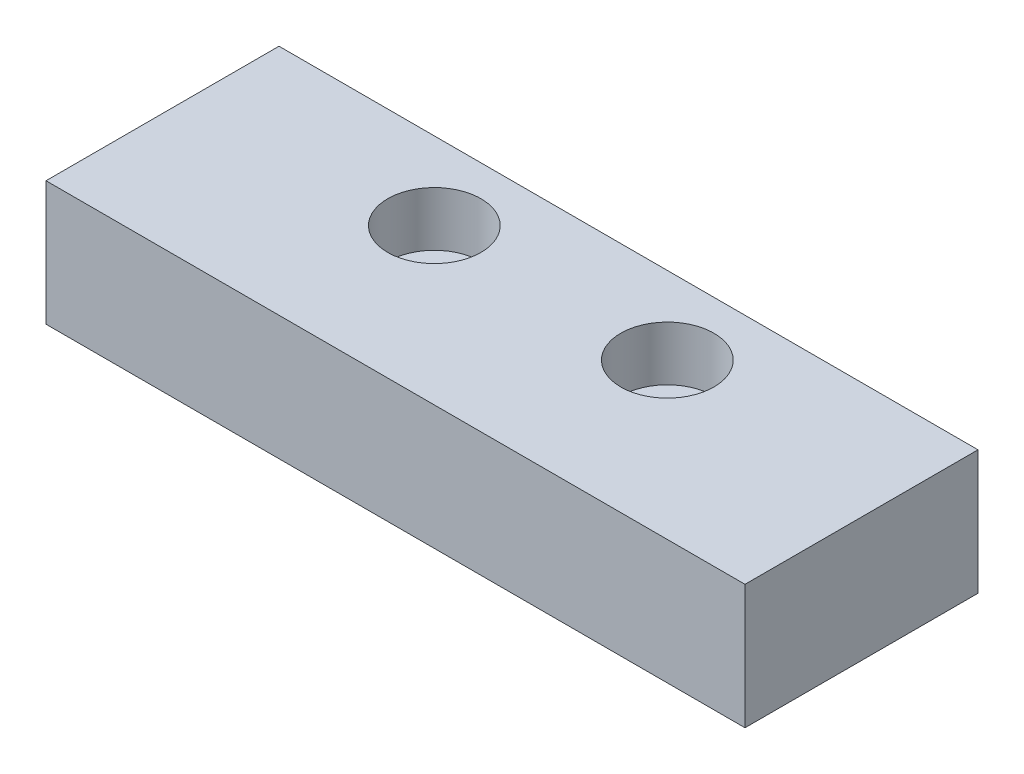
from build123d import *

# Parameters (mm, degrees)
SKETCH_1_W                = 45
SKETCH_1_H                = 10
EXTRUDE_1_DEPTH           = 8
HOLE_WIZARD_1_D           = 3.2
HOLE_WIZARD_1_CBORE_D     = 6
HOLE_WIZARD_1_CBORE_DEPTH = 3.5
SKETCH_4_W                = 45
SKETCH_4_H                = 8
EXTRUDE_2_DEPTH           = 5


with BuildPart() as part:
    # 草图1 → 凸台-拉伸1 (new body)
    with BuildSketch(Plane(origin=(0, 0, 0), x_dir=(1, 0, 0), z_dir=(0, 1, 0))):
        Rectangle(SKETCH_1_W, SKETCH_1_H)
    extrude(amount=EXTRUDE_1_DEPTH)

    # 打孔尺寸(%根据)开槽圆柱头螺钉的类型1 (through all)
    with Locations(Plane(origin=(0, 8, 0), x_dir=(1, 0, 0), z_dir=(0, 1, 0))):
        with Locations((-7.5, 0), (7.5, 0)):
            CounterBoreHole(HOLE_WIZARD_1_D / 2, HOLE_WIZARD_1_CBORE_D / 2, HOLE_WIZARD_1_CBORE_DEPTH)

    # 草图4 → 凸台-拉伸2 (add)
    with BuildSketch(Plane.XY.offset(5)):
        with Locations((0, 4)):
            Rectangle(SKETCH_4_W, SKETCH_4_H)
    extrude(amount=EXTRUDE_2_DEPTH)


solid = part.part
